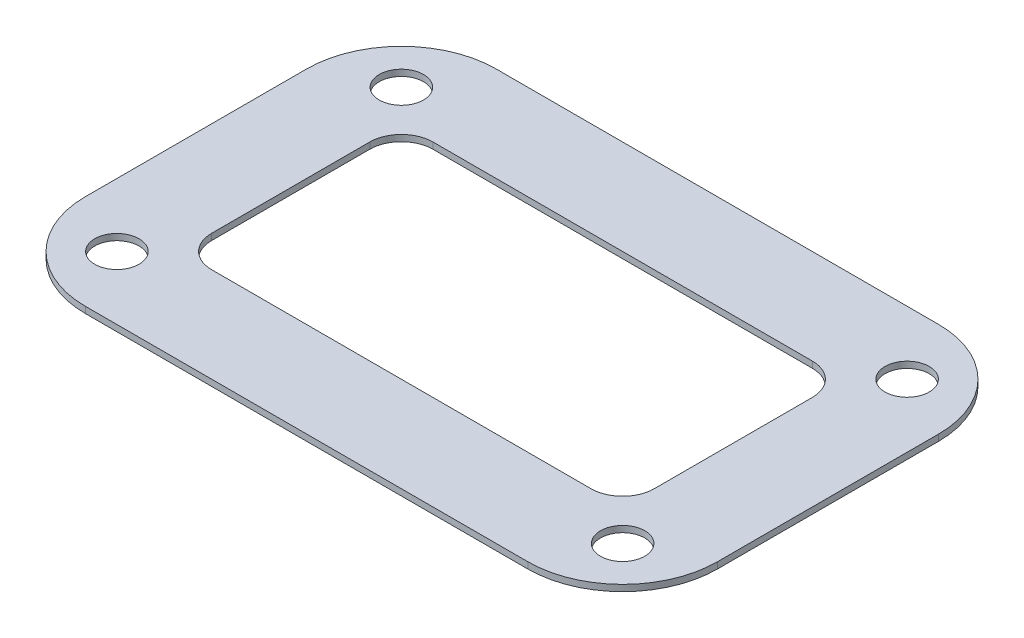
from build123d import *

# Parameters (mm, degrees)
BOSS_EXTRUDE1_DEPTH  = 1
CUT_EXTRUDE1_DEPTH   = 60.642686056
HOLE1_D              = 7
LPATTERN1_COUNT      = 2
LPATTERN1_PITCH      = 80
LPATTERN1_COUNT_DIR2 = 2
LPATTERN1_PITCH_DIR2 = 45


with BuildPart() as part:
    # Sketch1 → Boss-Extrude1 (new body)
    with BuildSketch(Plane(origin=(0, 0, 0), x_dir=(1, 0, 0), z_dir=(0, 1, 0))):
        with BuildLine():
            Line((-35, 32.5), (35, 32.5))
            ThreePointArc((35, 32.5), (45.606601718, 28.106601718), (50, 17.5))
            Line((50, 17.5), (50, -17.5))
            ThreePointArc((50, -17.5), (45.606601718, -28.106601718), (35, -32.5))
            Line((35, -32.5), (-35, -32.5))
            ThreePointArc((-35, -32.5), (-45.606601718, -28.106601718), (-50, -17.5))
            Line((-50, -17.5), (-50, 17.5))
            ThreePointArc((-50, 17.5), (-45.606601718, 28.106601718), (-35, 32.5))
        make_face()
    extrude(amount=BOSS_EXTRUDE1_DEPTH)

    # Sketch2 → Cut-Extrude1 (cut, through all)
    with BuildSketch(Plane(origin=(0, 1, 0), x_dir=(1, 0, 0), z_dir=(0, 1, 0))):
        with BuildLine():
            Line((-30, 17.5), (30, 17.5))
            ThreePointArc((30, 17.5), (33.535533906, 16.035533906), (35, 12.5))
            Line((35, 12.5), (35, -12.5))
            ThreePointArc((35, -12.5), (33.535533906, -16.035533906), (30, -17.5))
            Line((30, -17.5), (-30, -17.5))
            ThreePointArc((-30, -17.5), (-33.535533906, -16.035533906), (-35, -12.5))
            Line((-35, -12.5), (-35, 12.5))
            ThreePointArc((-35, 12.5), (-33.535533906, 16.035533906), (-30, 17.5))
        make_face()
    extrude(amount=-CUT_EXTRUDE1_DEPTH, mode=Mode.SUBTRACT)

    # Hole1 (through all)
    with Locations(Plane(origin=(-40, 1, -22.5), x_dir=(0, 0, 1), z_dir=(0, 1, 0))):
        with Locations((0, 0)):
            hole1 = Hole(HOLE1_D / 2)

    # LPattern1: Hole1 2 × 2
    with Locations(*[(i * LPATTERN1_PITCH, 0, j * LPATTERN1_PITCH_DIR2) for i in range(LPATTERN1_COUNT) for j in range(LPATTERN1_COUNT_DIR2) if (i, j) != (0, 0)]):
        add(hole1, mode=Mode.SUBTRACT)


solid = part.part
